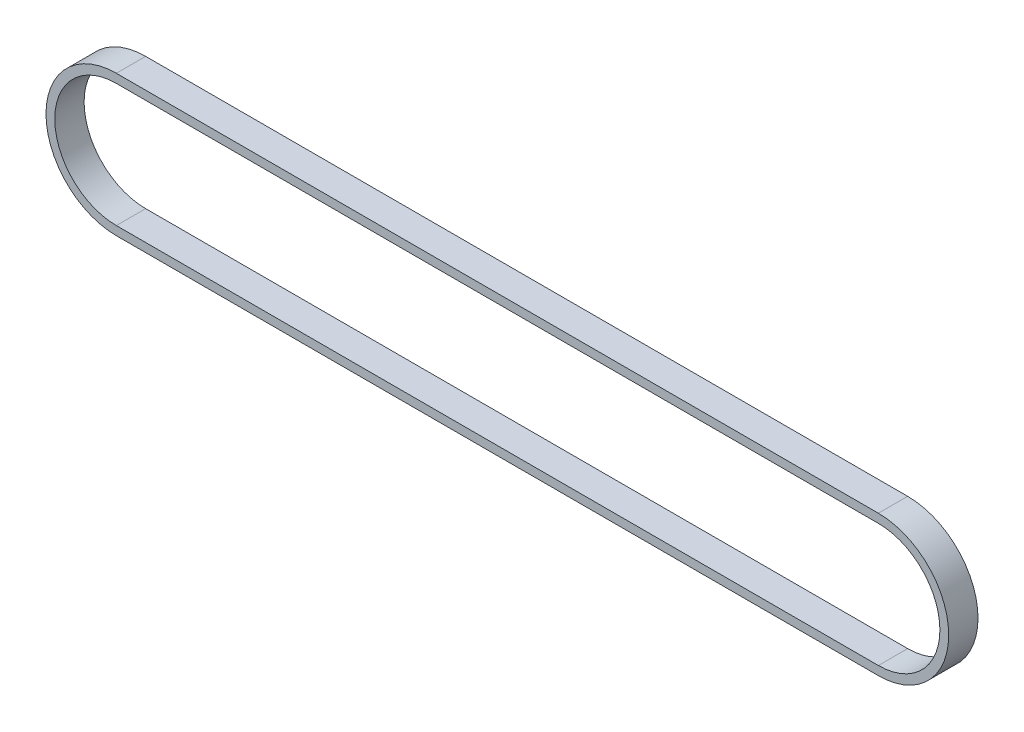
from build123d import *

# Parameters (mm, degrees)
BOSS_EXTRUDE1_DEPTH = 10
SHELL1_T            = -3


with BuildPart() as part:
    # Sketch2 → Boss-Extrude1 (new body)
    with BuildSketch(Plane.XY):
        with BuildLine():
            Line((0, 24), (-260, 24))
            ThreePointArc((-260, 24), (-284, 0), (-260, -24))
            Line((-260, -24), (0, -24))
            ThreePointArc((0, -24), (24, 0), (0, 24))
        make_face()
    extrude(amount=BOSS_EXTRUDE1_DEPTH)

    # Shell1
    shell1_openings = [part.faces().sort_by_distance(p)[0] for p in [
        (-130, 0, 10),
        (-130, 0, 0),
    ]]
    offset(amount=SHELL1_T, openings=shell1_openings, kind=Kind.INTERSECTION)


solid = part.part
